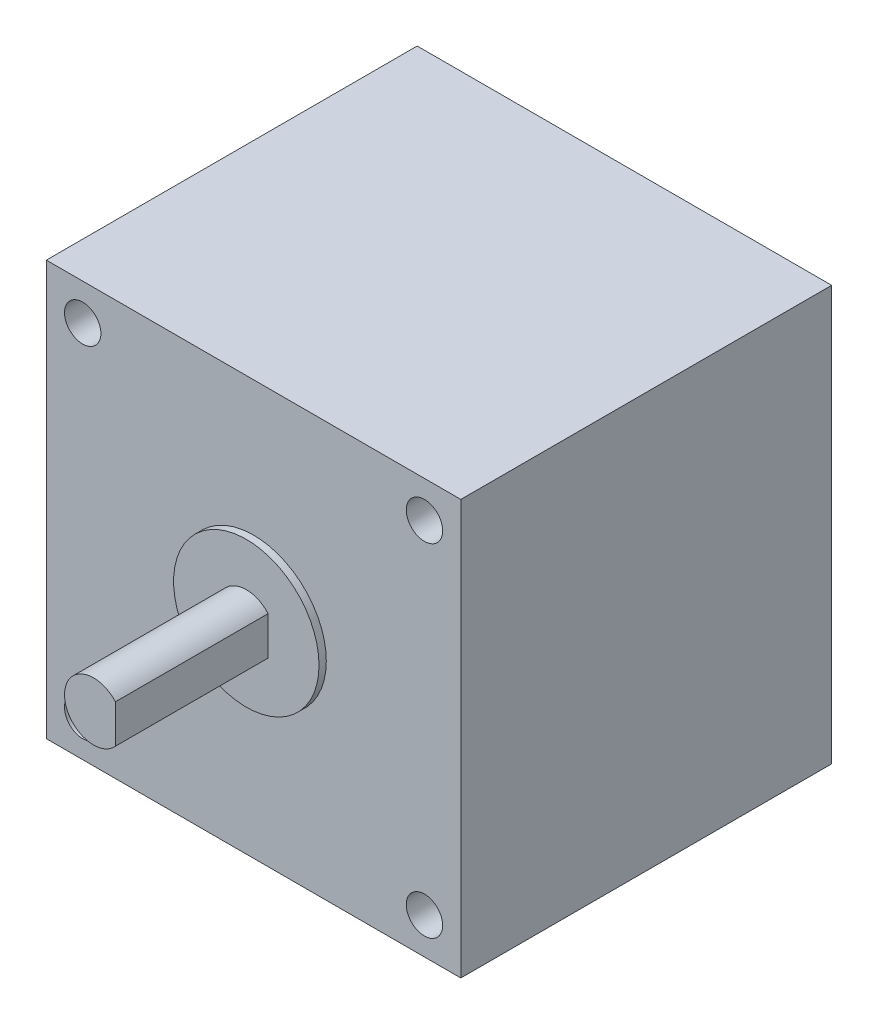
from build123d import *

# Parameters (mm, degrees)
SKETCH1_W           = 57
SKETCH1_H           = 57
BOSS_EXTRUDE1_DEPTH = 51
SKETCH2_R           = 2.5
CUT_EXTRUDE1_DEPTH  = 98
SKETCH4_R           = 10
BOSS_EXTRUDE2_DEPTH = 1
SKETCH5_R           = 4
BOSS_EXTRUDE3_DEPTH = 21
CUT_EXTRUDE2_DEPTH  = 21


with BuildPart() as part:
    # Sketch1 → Boss-Extrude1 (new body)
    with BuildSketch(Plane.XY):
        Rectangle(SKETCH1_W, SKETCH1_H)
    extrude(amount=BOSS_EXTRUDE1_DEPTH)

    # Sketch2 → Cut-Extrude1 (cut)
    with BuildSketch(Plane.XY.offset(51)):
        with Locations((-23.5, 23.5)):
            Circle(SKETCH2_R)
        with Locations((23.5, 23.5)):
            Circle(SKETCH2_R)
        with Locations((23.5, -23.5)):
            Circle(SKETCH2_R)
        with Locations((-23.5, -23.5)):
            Circle(SKETCH2_R)
    extrude(amount=-CUT_EXTRUDE1_DEPTH, mode=Mode.SUBTRACT)

    # Sketch4 → Boss-Extrude2 (add)
    with BuildSketch(Plane.XY.offset(51)):
        Circle(SKETCH4_R)
    extrude(amount=BOSS_EXTRUDE2_DEPTH)

    # Sketch5 → Boss-Extrude3 (add)
    with BuildSketch(Plane.XY.offset(52)):
        with Locations(Location((0, 0, 0), (0, 0, 180))):
            Circle(SKETCH5_R)
    extrude(amount=BOSS_EXTRUDE3_DEPTH)

    # Sketch6 → Cut-Extrude2 (cut)
    with BuildSketch(Plane.XY.offset(73)):
        Polygon((3, 101.241638907), (3, 2.645751311), (3, -2.645751311), (3, -101.241638907), (200.191775192, -101.241638907), (200.191775192, 101.241638907), align=None)
    extrude(amount=-CUT_EXTRUDE2_DEPTH, mode=Mode.SUBTRACT)


solid = part.part
